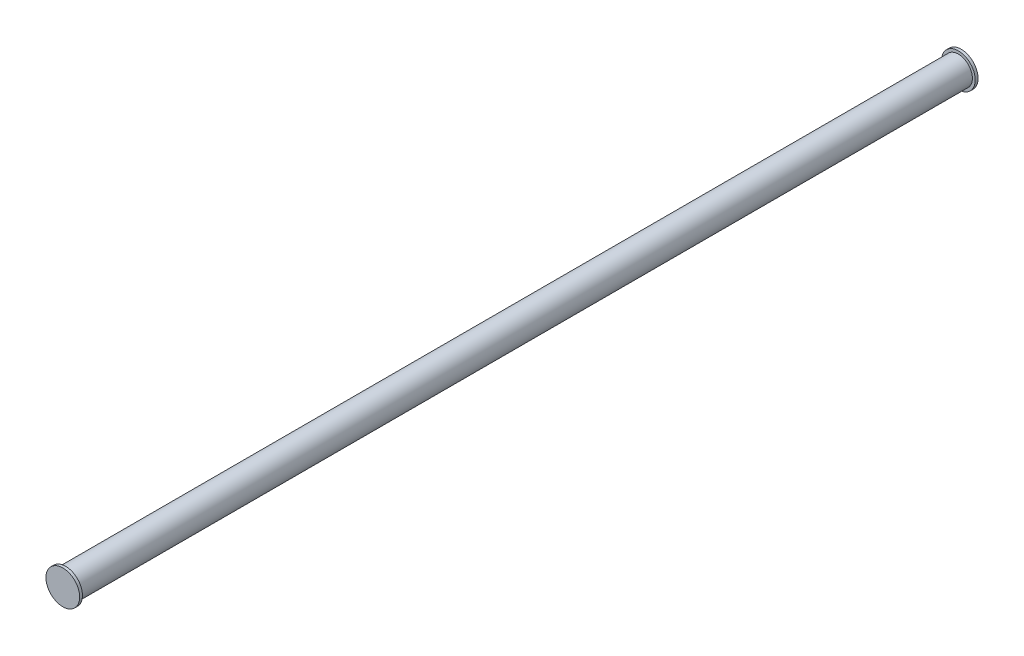
from build123d import *

# Parameters (mm, degrees)
SKETCH1_R           = 25
SKETCH1_R_2         = 24
BOSS_EXTRUDE1_DEPTH = 1590
SKETCH4_R           = 30
BOSS_EXTRUDE2_DEPTH = 5
BOSS_EXTRUDE3_START = 5
SKETCH5_R           = 30
BOSS_EXTRUDE3_DEPTH = 5


with BuildPart() as part:
    # Sketch1 → Boss-Extrude1 (new body)
    with BuildSketch(Plane.XY):
        Circle(SKETCH1_R)
        Circle(SKETCH1_R_2, mode=Mode.SUBTRACT)
    extrude(amount=BOSS_EXTRUDE1_DEPTH)

    # Sketch4 → Boss-Extrude2 (add)
    with BuildSketch(Plane(origin=(0, 0, 0), x_dir=(-1, 0, 0), z_dir=(0, 0, -1))):
        Circle(SKETCH4_R)
    extrude(amount=BOSS_EXTRUDE2_DEPTH)

    # Sketch5 → Boss-Extrude3 (add)
    with BuildSketch(Plane.XY.offset(1590).offset(BOSS_EXTRUDE3_START)):
        with Locations(Location((0, 0, 0), (0, 0, 180))):
            Circle(SKETCH5_R)
    extrude(amount=-BOSS_EXTRUDE3_DEPTH)


solid = part.part
